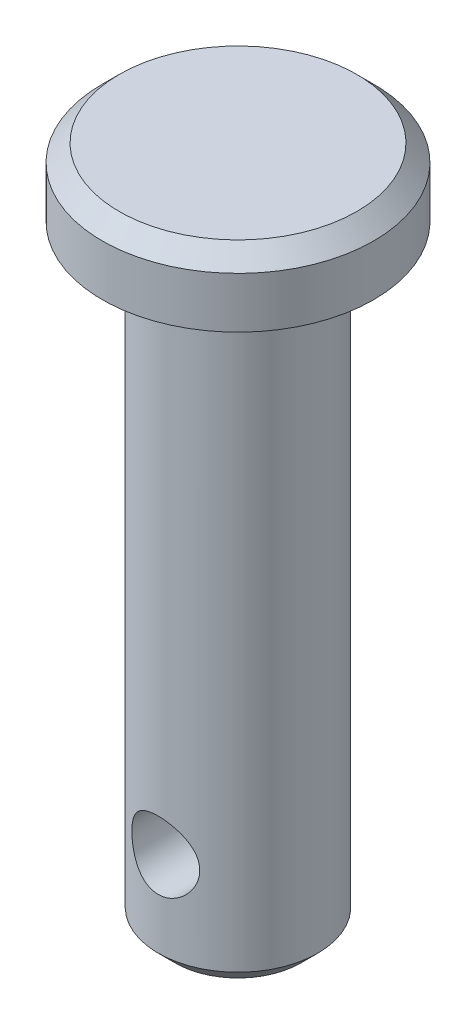
from build123d import *

# Parameters (mm, degrees)
FILLET1_R               = 0.5
CHAMFER1_SIZE           = 0.5
CUT_EXTRUDE1_DEPTH      = 21.784609691
CUT_EXTRUDE1_DEPTH_BACK = 21.784609691
SKETCH2_R               = 1


with BuildPart() as part:
    # Sketch1 → Revolve1 (revolve)
    with BuildSketch(Plane.XY):
        Polygon((0, 0), (4, 0), (4, -2), (2.35, -2), (2.35, -20), (0, -20), align=None)
    revolve(axis=Axis((0, -273.133875929, 0), (0, 1, 0)))

    # Fillet1
    fillet1_edges = [part.edges().sort_by_distance(p)[0] for p in [
        (-2.35, -2, 0),
    ]]
    fillet(fillet1_edges, radius=FILLET1_R)

    # Chamfer1
    chamfer1_edges = [part.edges().sort_by_distance(p)[0] for p in [
        (-2.35, -20, 0),
        (-4, 0, 0),
    ]]
    chamfer(chamfer1_edges, length=CHAMFER1_SIZE)

    # Sketch2 → Cut-Extrude1 (cut, two sides: drawn at the far end of the back side and taken through both)
    with BuildSketch(Plane.XY.offset(-CUT_EXTRUDE1_DEPTH_BACK)):
        with Locations((0, -17)):
            Circle(SKETCH2_R)
    extrude(amount=CUT_EXTRUDE1_DEPTH + CUT_EXTRUDE1_DEPTH_BACK, mode=Mode.SUBTRACT)


solid = part.part
